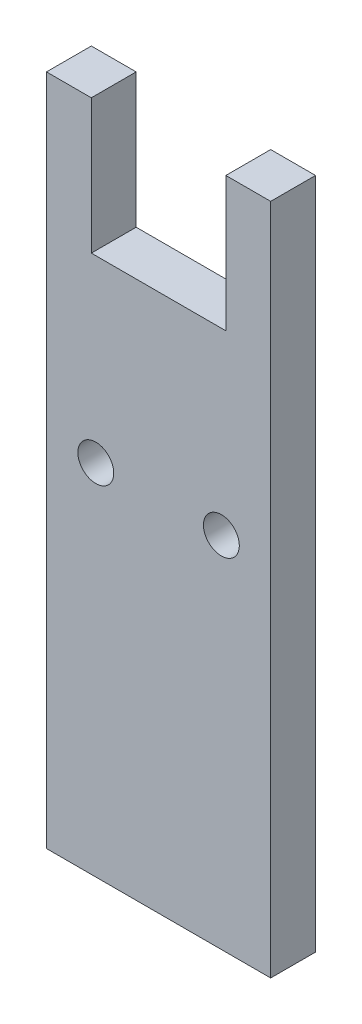
SolidWorks part; units mm, degrees
ref_plane "Front Plane" through (0, 0, 0) normal (0, 0, 1) x (1, 0, 0)
ref_plane "Top Plane" through (0, 0, 0) normal (0, 1, 0) x (1, 0, 0)
ref_plane "Right Plane" through (0, 0, 0) normal (1, 0, 0) x (0, 0, -1)
sketch "Sketch1" plane through (0, 0, 0) normal (0, 0, 1) x (1, 0, 0)
  line L1 (-25, -75) -> (25, -75)
  line L2 (-25, -75) -> (-25, 75)
  line L3 (-25, 75) -> (25, 75)
  line L4 (25, -75) -> (25, 75)
  line L5 (-25, -75) -> (25, 75) construction
  line L6 (-25, 75) -> (25, -75) construction
  point P0 (0, 0)
  dimension "D1" = 50
  dimension "D2" = 150
extrude "Boss-Extrude1" add sketch "Sketch1" along normal blind 10
sketch "Sketch2" plane through (0, 0, 10) normal (0, 0, 1) x (1, 0, 0)
  line L0 (25, 75) -> (-25, 75) construction
  line L1 (-15, 75) -> (15, 75)
  line L2 (-15, 75) -> (-15, 45)
  line L3 (-15, 45) -> (15, 45)
  line L4 (15, 75) -> (15, 45)
  line L5 (0, 0) -> (0, 45) construction
  dimension "D1" = 30
  dimension "D2" = 30
extrude "Cut-Extrude1" cut sketch "Sketch2" against normal blind 10
sketch "Sketch3" plane through (0, 0, 10) normal (0, 0, 1) x (1, 0, 0)
  line L0 (-25, -75) -> (25, -75) construction
  line L1 (0, 0) -> (0, -75) construction
  circle A0 centre (-14, 5) radius 4
  circle A1 centre (14, 5) radius 4
  dimension "D2" = 8
  dimension "D3" = 28
  dimension "D1" = 80
extrude "Cut-Extrude2" cut sketch "Sketch3" against normal through all
